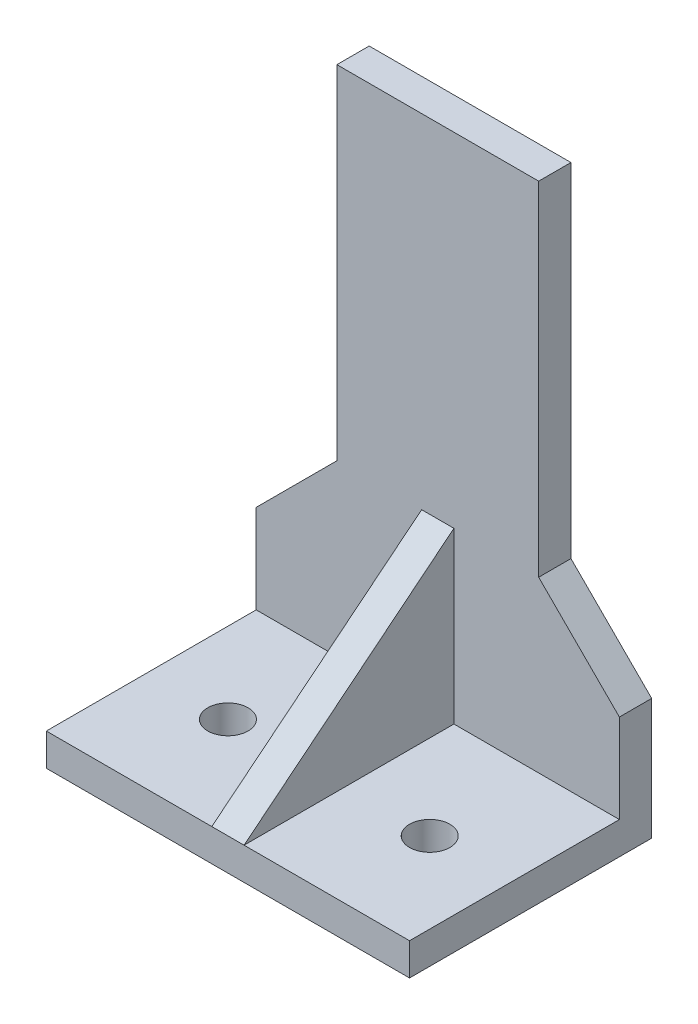
from build123d import *
from build123d.topology import SkipClean

# Parameters (mm, degrees)
EXTRUDE_2_DEPTH      = 8
SKETCH_2_W           = 90
SKETCH_2_H           = 8
EXTRUDE_3_DEPTH      = 52
EXTRUDE_4_DEPTH      = 4
EXTRUDE_4_DEPTH_BACK = 4
CUT_EXTRUDE_2_DEPTH  = 18
SKETCH_6_R           = 5
CUT_EXTRUDE_3_DEPTH  = 10
SKETCH_8_R           = 5
CUT_EXTRUDE_4_DEPTH  = 10
EXTRUDE_6_DEPTH      = 8


with BuildPart() as part:
    # 草图1 → 凸台-拉伸2 (new body)
    with BuildSketch(Plane.XY):
        Polygon((0, 0), (90, 0), (90, 30), (70, 50), (70, 135), (45, 135), (20, 135), (20, 50), (0, 30), align=None)
    extrude(amount=EXTRUDE_2_DEPTH)

    # 草图2 → 凸台-拉伸3 (add)
    with BuildSketch(Plane.XY.offset(8)):
        with Locations((45, 4)):
            Rectangle(SKETCH_2_W, SKETCH_2_H)
    extrude(amount=EXTRUDE_3_DEPTH)

    # 草图4 → 凸台-拉伸4 (add, two sides: drawn at the far end of the back side and taken through both)
    with BuildSketch(Plane(origin=(45, 0, 0), x_dir=(0, 0, -1), z_dir=(1, 0, 0)).offset(-EXTRUDE_4_DEPTH_BACK)):
        Polygon((-8, 8), (-8, 50), (-60, 8), align=None)
    extrude(amount=EXTRUDE_4_DEPTH + EXTRUDE_4_DEPTH_BACK)

    # 草图5 → 切除-拉伸2 (cut)
    with BuildSketch(Plane(origin=(0, 8, 0), x_dir=(1, 0, 0), z_dir=(0, 1, 0))):
        with BuildLine():
            ThreePointArc((70, -35), (65, -30), (60, -35))
            Line((60, -35), (65, -35))
            Line((65, -35), (70, -35))
        make_face()
        with BuildLine():
            Line((65, -35), (60, -35))
            ThreePointArc((60, -35), (65, -40), (70, -35))
            Line((70, -35), (65, -35))
        make_face()
        with BuildLine():
            Line((20, -35), (25, -35))
            Line((25, -35), (30, -35))
            ThreePointArc((30, -35), (25, -30), (20, -35))
        make_face()
        with BuildLine():
            Line((30, -35), (25, -35))
            Line((25, -35), (20, -35))
            ThreePointArc((20, -35), (25, -40), (30, -35))
        make_face()
    extrude(amount=-CUT_EXTRUDE_2_DEPTH, mode=Mode.SUBTRACT)

    # 草图6 → 切除-拉伸3 (cut)
    with BuildSketch(Plane(origin=(0, 8, 0), x_dir=(1, 0, 0), z_dir=(0, 1, 0))):
        with Locations((20, -35)):
            Circle(SKETCH_6_R)
    extrude(amount=-CUT_EXTRUDE_3_DEPTH, mode=Mode.SUBTRACT)

    # 草图8 → 切除-拉伸4 (cut)
    with BuildSketch(Plane(origin=(0, 8, 0), x_dir=(1, 0, 0), z_dir=(0, 1, 0))):
        with Locations((70, -35)):
            Circle(SKETCH_8_R)
        with Locations((65, -35)):
            Circle(SKETCH_8_R)
    extrude(amount=-CUT_EXTRUDE_4_DEPTH, mode=Mode.SUBTRACT)

    # 草图9 → 凸台-拉伸6 (add)
    with SkipClean():  # the faces are left unmerged after this step: merging them gives an invalid solid
        with BuildSketch(Plane(origin=(0, 8, 0), x_dir=(1, 0, 0), z_dir=(0, 1, 0))):
            with BuildLine():
                ThreePointArc((22.5, -30.669872981), (25, -35), (22.5, -39.330127019))
                ThreePointArc((22.5, -39.330127019), (30, -35), (22.5, -30.669872981))
            make_face()
            with BuildLine():
                ThreePointArc((67.5, -39.330127019), (65, -35), (67.5, -30.669872981))
                ThreePointArc((67.5, -30.669872981), (60, -35), (67.5, -39.330127019))
            make_face()
        extrude(amount=-EXTRUDE_6_DEPTH)


solid = part.part
